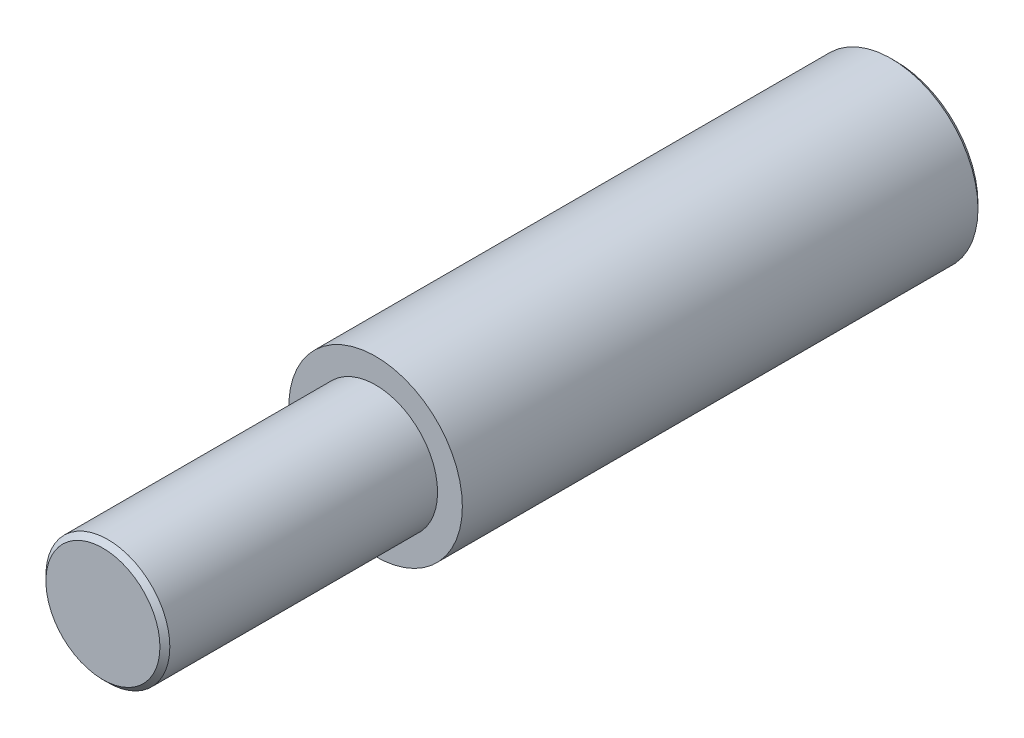
from build123d import *

# Parameters (mm, degrees)
SKETCH1_R           = 17.5
BOSS_EXTRUDE1_DEPTH = 105
SKETCH2_R           = 12.5
BOSS_EXTRUDE2_DEPTH = 55
CHAMFER1_SIZE       = 1


with BuildPart() as part:
    # Sketch1 → Boss-Extrude1 (new body)
    with BuildSketch(Plane.XY):
        Circle(SKETCH1_R)
    extrude(amount=BOSS_EXTRUDE1_DEPTH)

    # Sketch2 → Boss-Extrude2 (add)
    with BuildSketch(Plane.XY.offset(105)):
        Circle(SKETCH2_R)
    extrude(amount=BOSS_EXTRUDE2_DEPTH)

    # Chamfer1
    chamfer1_edges = [part.edges().sort_by_distance(p)[0] for p in [
        (-17.5, 0, 0),
        (-12.5, 0, 160),
    ]]
    chamfer(chamfer1_edges, length=CHAMFER1_SIZE)


solid = part.part
